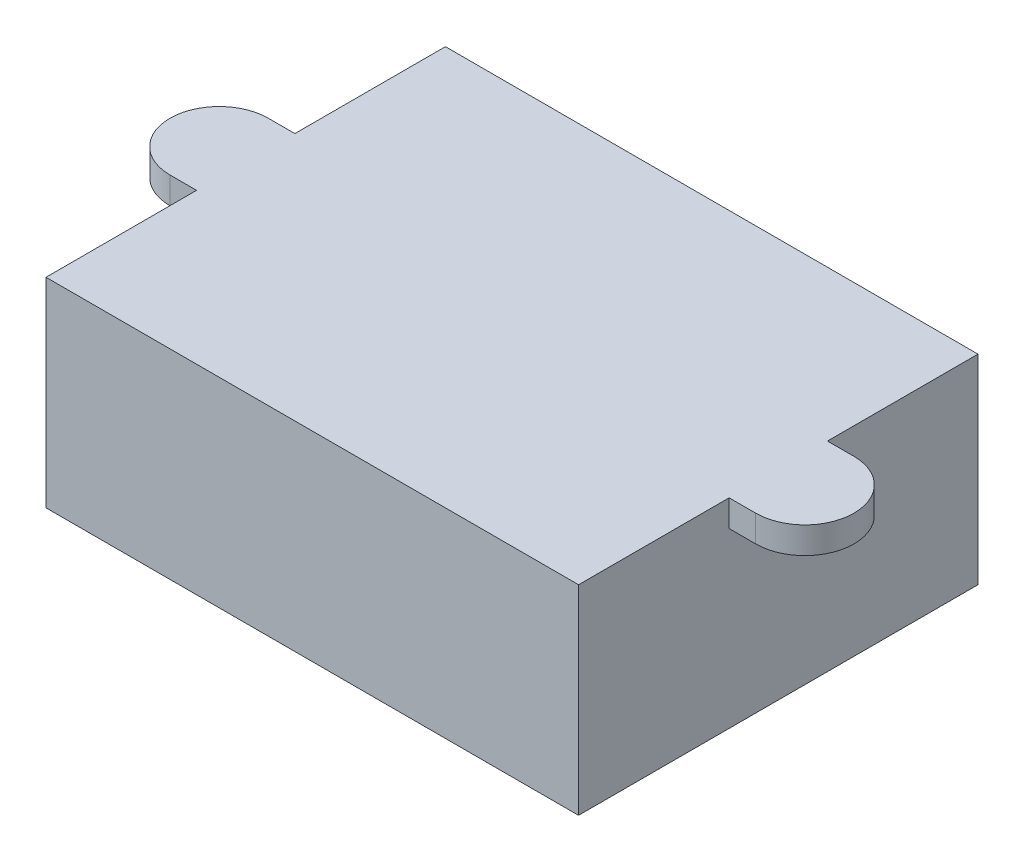
SolidWorks part; units mm, degrees
ref_plane "Front Plane" through (0, 0, 0) normal (0, 0, 1) x (1, 0, 0)
ref_plane "Top Plane" through (0, 0, 0) normal (0, 1, 0) x (1, 0, 0)
ref_plane "Right Plane" through (0, 0, 0) normal (1, 0, 0) x (0, 0, -1)
sketch "Sketch1" plane through (0, 0, 0) normal (0, 1, 0) x (1, 0, 0)
  line L1 (-20, 15) -> (20, 15)
  line L2 (-20, 15) -> (-20, -15)
  line L3 (-20, -15) -> (20, -15)
  line L4 (20, 15) -> (20, -15)
  line L5 (-20, 15) -> (20, -15) construction
  line L6 (-20, -15) -> (20, 15) construction
  point P0 (0, 0)
  dimension "D1" = 30
  dimension "D2" = 40
extrude "Boss-Extrude1" add sketch "Sketch1" along normal blind 15
sketch "Sketch2" plane through (0, 15, 0) normal (0, 1, 0) x (1, 0, 0)
  line L0 (-21.9958, 0) -> (21.9958, 0) construction
  line L1 (-21.9958, 3.6916) -> (21.9958, 3.6916)
  line L2 (-21.9958, -3.6916) -> (21.9958, -3.6916)
  arc A0 (-21.9958, 3.6916) -> (-21.9958, -3.6916) centre (-21.9958, 0) ccw
  arc A1 (21.9958, -3.6916) -> (21.9958, 3.6916) centre (21.9958, 0) ccw
  point P2 (0, 0)
extrude "Boss-Extrude2" add sketch "Sketch2" against normal blind 2
sketch "Sketch3" plane through (0, 0, 0) normal (0, -1, 0) x (1, 0, 0)
  circle A0 centre (-15.1141, 6.9511) radius 1.4088
  circle A1 centre (-8.0715, 6.9511) radius 1.4088
  circle A2 centre (-15.1141, -6.4481) radius 1.4088
  circle A3 centre (-8.0715, -6.4481) radius 1.4088
extrude "Cut-Extrude1" cut sketch "Sketch3" against normal blind 5
